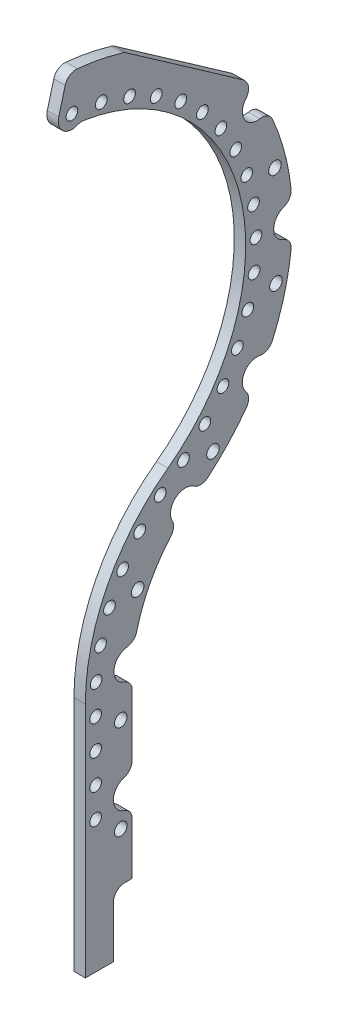
SolidWorks part; units mm, degrees
material "Thornel Mat VMA"
ref_plane "前视基准面" through (0, 0, 0) normal (0, 0, 1) x (1, 0, 0)
ref_plane "上视基准面" through (0, 0, 0) normal (0, 1, 0) x (1, 0, 0)
ref_plane "右视基准面" through (0, 0, 0) normal (1, 0, 0) x (0, 0, -1)
sketch "弹链路径" plane through (0, 0, 0) normal (1, 0, 0) x (0, 0, -1)
  line L0 (0, -41.5) -> (0, 0)
  line L1 (0, 80) -> (6.1652, 79.4606)
  line L2 (0, 80) -> (3.3166, 80) construction
  line L3 (7.1501, 90.7176) -> (5.1803, 68.2036) construction
  arc A0 (18.3088, 36.2295) -> (0, 0) centre (45, 0) ccw
  arc A1 (18.3088, 36.2295) -> (6.1652, 79.4606) centre (4.0735, 55.5519) ccw
  point P11 (6.1652, 79.4606)
  dimension "D1" = 45
  dimension "D2" = 24
  dimension "D3" = 5
  dimension "D4" = 80
  dimension "D5" = 121.5
  dimension "D6" = 22.6
sketch "螺纹孔位" plane through (0, 0, 0) normal (1, 0, 0) x (0, 0, -1)
  line L0 (4.0735, 55.5519) -> (39.5805, 76.0519) construction
  line L1 (4.0735, 55.5519) -> (45.0735, 55.5519) construction
  line L2 (4.0735, 55.5519) -> (39.5805, 35.0519) construction
  line L3 (45, 0) -> (0, 0) construction
  line L4 (-17, -17) -> (17, -17) construction
  line L5 (0, -41.5) -> (0, 0) construction
  line L6 (-15.3402, 14.25) -> (17.1065, 2.4404) construction
  line L7 (2.9189, 45.5322) -> (27.0019, 21.4492) construction
  line L8 (45, 0) -> (27.0019, 21.4492) construction
  line L9 (45, 0) -> (17.1065, 2.4404) construction
  arc A0 (39.5805, 76.0519) -> (39.5805, 35.0519) centre (4.0735, 55.5519) cw construction
  circle A1 centre (39.5805, 76.0519) radius 1.5
  circle A2 centre (39.5805, 35.0519) radius 1.5
  circle A3 centre (45.0735, 55.5519) radius 1.5
  circle A4 centre (-17, -17) radius 1.5
  circle A5 centre (17, -17) radius 1.5
  arc A6 (-15.3402, 14.25) -> (2.9189, 45.5322) centre (45, 0) cw construction
  arc A7 (17.1065, 2.4404) -> (27.0019, 21.4492) centre (45, 0) cw construction
  circle A8 centre (-15.3402, 14.25) radius 1.5
  circle A9 centre (2.9189, 45.5322) radius 1.5
  circle A10 centre (27.0019, 21.4492) radius 1.5
  circle A11 centre (17.1065, 2.4404) radius 1.5
  point P10 (0, -17)
  dimension "D1" = 41
  dimension "D3" = 62
  dimension "D4" = 28
  dimension "D11" = 3
  dimension "D2" = 30
  dimension "D5" = 175
  dimension "D6" = 165
  dimension "D7" = 5
  dimension "D8" = 45
  dimension "D9" = 17
  dimension "D10" = 34
sketch "草图3" plane through (0, 0, 0) normal (1, 0, 0) x (0, 0, -1)
  line L4 (4.0735, 55.5519) -> (45.0735, 55.5519) construction
  line L5 (4.0735, 55.5519) -> (45.0735, 55.5519) construction
  line L6 (17.7, -14.496) -> (17.7, -0.091)
  line L7 (19.5, 0) -> (19.5, -25) construction
  line L8 (13.9, 0) -> (13.9, -25) construction
  line L9 (13.9, -25) -> (19.5, -25) construction
  line L10 (17.7, -30.5) -> (17.7, 0) construction
  line L11 (27.986, 89.7026) -> (38.1572, 82.5807) construction
  line L12 (27.986, 89.7026) -> (24.774, 85.1153) construction
  line L13 (17.7, -30.5) -> (17.7, -19.504)
  line L15 (37.3155, 80.7284) -> (16.3622, 95.4001)
  line L16 (17.7, -30.5) -> (14.4, -30.5)
  line L17 (34.253, 78.4781) -> (24.774, 85.1153) construction
  line L18 (15.7, -30.5) -> (15.7, 0) construction
  line L19 (35.9077, 79.2727) -> (25.6917, 86.426) construction
  line L20 (14.4, -30.5) -> (14.4, -41.5)
  line L21 (14.4, -41.5) -> (9.5, -41.5)
  line L22 (9.5, -41.5) -> (9.5, 0)
  line L23 (37.3155, 80.7284) -> (26.8388, 88.0643) construction
  line L24 (6.3989, 97.1871) -> (4.8318, 91.3388)
  line L25 (11.3, -13.1623) -> (11.3, -18.3623) construction
  line L26 (7.1501, 90.7176) -> (12.2828, 89.8841) construction
  line L27 (12.2828, 89.8841) -> (17.2374, 88.3056) construction
  line L28 (17.2374, 88.3056) -> (21.9064, 86.0163) construction
  line L29 (21.9064, 86.0163) -> (26.1884, 83.0659) construction
  line L30 (26.1884, 83.0659) -> (29.9905, 79.5185) construction
  line L31 (29.9905, 79.5185) -> (33.2302, 75.4511) construction
  line L32 (33.2302, 75.4511) -> (35.8372, 70.9518) construction
  line L33 (35.8372, 70.9518) -> (37.7549, 66.1183) construction
  line L34 (37.7549, 66.1183) -> (38.9418, 61.0556) construction
  line L35 (38.9418, 61.0556) -> (39.372, 55.8734) construction
  line L36 (39.372, 55.8734) -> (39.0362, 50.6843) construction
  line L37 (39.0362, 50.6843) -> (37.9418, 45.6007) construction
  line L38 (37.9418, 45.6007) -> (36.1124, 40.7332) construction
  line L39 (36.1124, 40.7332) -> (33.5878, 36.1871) construction
  line L40 (33.5878, 36.1871) -> (30.4227, 32.0613) construction
  line L41 (30.4227, 32.0613) -> (26.6858, 28.4453) construction
  line L42 (26.6858, 28.4453) -> (22.6236, 25.199) construction
  line L43 (22.6236, 25.199) -> (19.0133, 21.4565) construction
  line L44 (19.0133, 21.4565) -> (16.0218, 17.2032) construction
  line L45 (16.0218, 17.2032) -> (13.7201, 12.5404) construction
  line L46 (13.7201, 12.5404) -> (12.1633, 7.5789) construction
  line L47 (12.1633, 7.5789) -> (11.3882, 2.437) construction
  line L48 (11.3882, 2.437) -> (11.3, -2.7623) construction
  line L49 (11.3, -2.7623) -> (11.3, -7.9623) construction
  line L50 (11.3, -7.9623) -> (11.3, -13.1623) construction
  line L51 (11.3, 0) -> (11.3, -41.5) construction
  line L52 (35.9077, 79.2727) -> (25.6917, 86.426) construction
  circle A1 centre (39.5805, 76.0519) radius 1.5 construction
  circle A2 centre (45.0735, 55.5519) radius 1.5 construction
  circle A3 centre (39.5805, 35.0519) radius 1.5 construction
  circle A4 centre (27.0019, 21.4492) radius 1.5 construction
  circle A5 centre (11.3, -18.3623) radius 1.025
  circle A7 centre (17.1065, 2.4404) radius 1.5 construction
  circle A8 centre (17, -17) radius 1.5 construction
  arc A9 (18.1307, 4.8302) -> (17.7, -0.091) centre (17.1065, 2.4404) ccw
  circle A10 centre (39.5805, 76.0519) radius 1.5 construction
  circle A11 centre (45.0735, 55.5519) radius 1.5 construction
  circle A12 centre (39.5805, 35.0519) radius 1.5 construction
  circle A13 centre (27.0019, 21.4492) radius 1.5 construction
  circle A16 centre (17.1065, 2.4404) radius 1.5 construction
  circle A17 centre (17, -17) radius 1.5 construction
  arc A25 (29.875, 20.5301) -> (19.5, 0) centre (45, 0) ccw construction
  arc A29 (26.5534, 25.0386) -> (13.9, 0) centre (45, 0) ccw construction
  arc A31 (25.6318, 19.2396) -> (18.1307, 4.8302) centre (45, 0) ccw
  arc A32 (26.5534, 25.0386) -> (34.253, 78.4781) centre (4.0735, 55.5519) ccw construction
  arc A34 (29.4094, 22.4312) -> (38.8584, 32.5542) centre (4.0735, 55.5519) ccw
  arc A35 (29.875, 20.5301) -> (38.1572, 82.5807) centre (4.0735, 55.5519) ccw construction
  arc A36 (17.7, -14.496) -> (17.7, -19.504) centre (17, -17) ccw
  arc A38 (27.621, 23.5894) -> (15.7, 0) centre (45, 0) ccw construction
  arc A39 (27.621, 23.5894) -> (35.9077, 79.2727) centre (4.0735, 55.5519) ccw construction
  circle A44 centre (15.7, -22) radius 1.1
  circle A45 centre (15.7, -5.5) radius 1.1
  circle A46 centre (18.6561, 12.8254) radius 1.1
  circle A47 centre (30.4428, 83.0992) radius 1.1 construction
  circle A48 centre (42.6935, 64.749) radius 1.1
  circle A49 centre (31.8415, 27.1789) radius 1.1
  circle A50 centre (42.866, 47.1124) radius 1.1
  arc A51 (29.4094, 22.4312) -> (25.6318, 19.2396) centre (27.0019, 21.4492) ccw
  arc A52 (41.3826, 36.9261) -> (38.8584, 32.5542) centre (39.5805, 35.0519) ccw
  arc A53 (45.697, 58.0761) -> (45.697, 53.0278) centre (45.0735, 55.5519) ccw
  arc A54 (38.8584, 78.5497) -> (41.3826, 74.1778) centre (39.5805, 76.0519) ccw
  arc A56 (28.8073, 21.9792) -> (17.7, 0) centre (45, 0) ccw construction
  arc A57 (28.8073, 21.9792) -> (37.3155, 80.7284) centre (4.0735, 55.5519) ccw construction
  arc A58 (41.3826, 36.9261) -> (45.697, 53.0278) centre (4.0735, 55.5519) ccw
  arc A59 (45.697, 58.0761) -> (41.3826, 74.1778) centre (4.0735, 55.5519) ccw
  arc A60 (38.8584, 78.5497) -> (37.3155, 80.7284) centre (4.0735, 55.5519) ccw
  circle A61 centre (7.1501, 90.7176) radius 1.025
  arc A63 (23.9436, 28.5811) -> (8.5302, 88.7542) centre (4.0735, 55.5519) ccw
  arc A64 (23.9436, 28.5811) -> (9.5, 0) centre (45, 0) ccw
  arc A65 (4.8318, 91.3388) -> (8.5302, 88.7542) centre (7.1501, 90.7176) ccw
  arc A66 (16.3622, 95.4001) -> (6.3989, 97.1871) centre (4.0735, 55.5519) ccw
  arc A67 (25.0112, 27.1319) -> (11.3, 0) centre (45, 0) ccw construction
  arc A68 (25.0112, 27.1319) -> (6.1278, 90.7921) centre (4.0735, 55.5519) ccw construction
  circle A69 centre (12.2828, 89.8841) radius 1.025
  circle A70 centre (17.2374, 88.3056) radius 1.025
  circle A71 centre (21.9064, 86.0163) radius 1.025
  circle A72 centre (26.1884, 83.0659) radius 1.025
  circle A73 centre (29.9905, 79.5185) radius 1.025
  circle A74 centre (33.2302, 75.4511) radius 1.025
  circle A75 centre (35.8372, 70.9518) radius 1.025
  circle A76 centre (37.7549, 66.1183) radius 1.025
  circle A77 centre (38.9418, 61.0556) radius 1.025
  circle A78 centre (39.372, 55.8734) radius 1.025
  circle A79 centre (39.0362, 50.6843) radius 1.025
  circle A80 centre (37.9418, 45.6007) radius 1.025
  circle A81 centre (36.1124, 40.7332) radius 1.025
  circle A82 centre (33.5878, 36.1871) radius 1.025
  circle A83 centre (30.4227, 32.0613) radius 1.025
  circle A84 centre (26.6858, 28.4453) radius 1.025
  circle A85 centre (22.6236, 25.199) radius 1.025
  circle A86 centre (19.0133, 21.4565) radius 1.025
  circle A87 centre (16.0218, 17.2032) radius 1.025
  circle A88 centre (13.7201, 12.5404) radius 1.025
  circle A89 centre (12.1633, 7.5789) radius 1.025
  circle A90 centre (11.3882, 2.437) radius 1.025
  circle A91 centre (11.3, -2.7623) radius 1.025
  circle A92 centre (11.3, -7.9623) radius 1.025
  circle A93 centre (11.3, -13.1623) radius 1.025
  point P46 (0, 80)
  dimension "D3" = 2.05
  dimension "D5" = 2.2
  dimension "D6" = 25.5
  dimension "D7" = 31.1
  dimension "D10" = 55
  dimension "D16" = 13.5
  dimension "D2" = 5.2
  dimension "D13" = 4.8
  dimension "D20" = 11.3
  dimension "D22" = 5.2
  dimension "D24" = 11.5
  dimension "D30" = 75
  dimension "D4" = 5
  dimension "D8" = 24
  dimension "D9" = 35
  dimension "D11" = 1.8
  dimension "D12" = 2
  dimension "D14" = 5.6
  dimension "D17" = 11
  dimension "D18" = 3.3
  dimension "D19" = 3
  dimension "D21" = 1.8
  dimension "D23" = 5.2
  dimension "D25" = 10.5
  dimension "D26" = 7.5
  dimension "D27" = 12.5
  dimension "D28" = 9.5
  dimension "D29" = 5.8
  dimension "D15" = 2
extrude "凸台-拉伸1" add sketch "草图3" along normal mid plane 2 contours A51 | L8 L9 L7 A25 A35 L11 L12 L17 A32 A29 | A47 | A48 | A50 | A49 | A46 | A45 | A44
fillet "R2 圆角1" radius 2 17 edges at (0, 88.7542, -8.5302) (0, -30.5, -14.4) (0, -19.504, -17.7) (0, -14.496, -17.7) (0, 19.2396, -25.6318) (0, 22.4312, -29.4094) (0, 32.5542, -38.8584) (0, 36.9261, -41.3826) (0, 53.0278, -45.697) (0, 58.0761, -45.697) (0, 74.1778, -41.3826) (0, 78.5497, -38.8584) (0, 80.7284, -37.3155) (0, 95.4001, -16.3622) (0, 97.1871, -6.3989) (0, -0.091, -17.7) (0, 4.8302, -18.1307)
